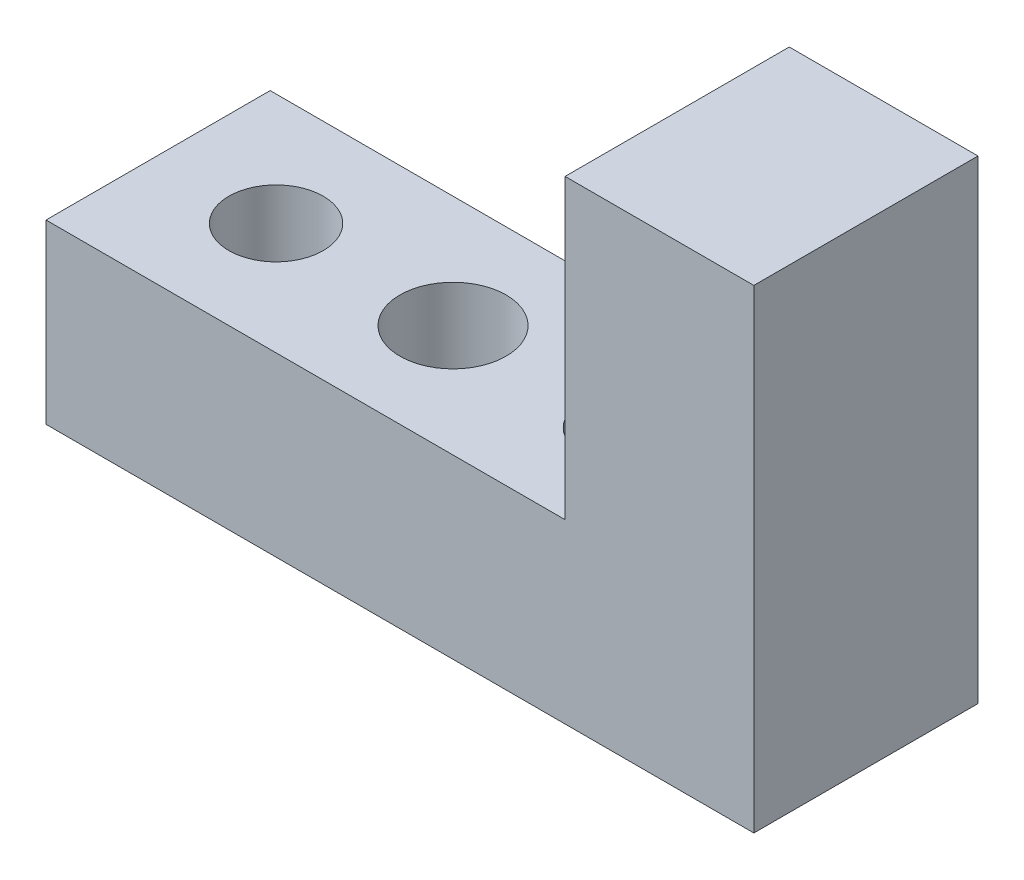
SolidWorks part; units mm, degrees
ref_plane "Front Plane" through (0, 0, 0) normal (0, 0, 1) x (1, 0, 0)
ref_plane "Top Plane" through (0, 0, 0) normal (0, 1, 0) x (1, 0, 0)
ref_plane "Right Plane" through (0, 0, 0) normal (1, 0, 0) x (0, 0, -1)
sketch "Sketch1" plane through (0, 0, 0) normal (0, 0, 1) x (1, 0, 0)
  line L0 (0, 0) -> (60, 0)
  line L1 (60, 0) -> (60, 40.2)
  line L2 (60, 40.2) -> (44, 40.2)
  line L3 (44, 40.2) -> (44, 15)
  line L4 (44, 15) -> (0, 15)
  line L5 (0, 15) -> (0, 0)
  dimension "D1" = 60
  dimension "D2" = 15
  dimension "D3" = 40.2
  dimension "D4" = 44
extrude "Boss-Extrude1" add sketch "Sketch1" along normal blind 19
ref_plane "Plane1" through (0, 0, 0) normal (0, -1, 0) x (-1, 0, 0)
sketch "Sketch2" plane through (0, 0, 0) normal (0, -1, 0) x (-1, 0, 0)
  line L0 (0, -9.5) -> (-60, -9.5) construction
  line L1 (0, -19) -> (0, 0) construction
  line L2 (-60, -19) -> (-60, 0) construction
  circle A0 centre (-10, -9.5) radius 4
  circle A1 centre (-25, -9.5) radius 4.5
  circle A2 centre (-40, -9.5) radius 4
  dimension "D1" = 10
  dimension "D2" = 15
  dimension "D3" = 15
extrude "Cut-Extrude1" cut sketch "Sketch2" against normal blind 15
